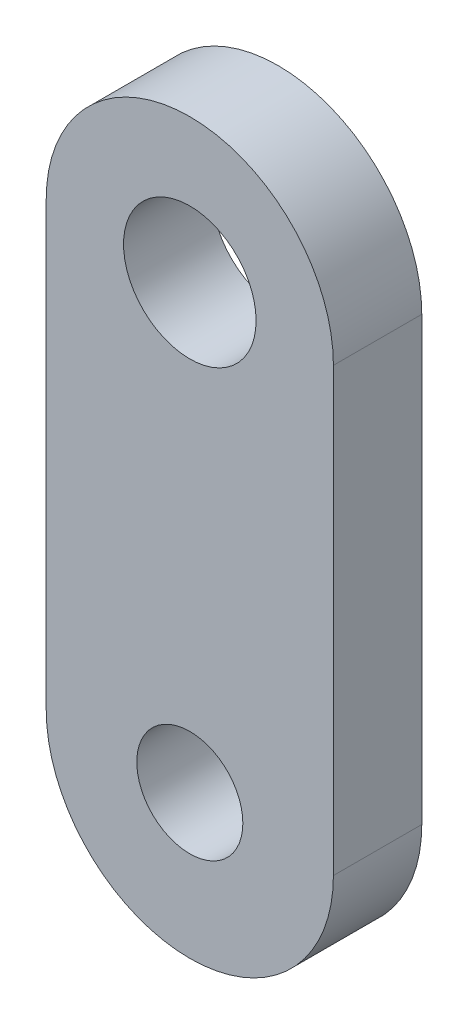
from build123d import *

# Parameters (mm, degrees)
SKETCH1_R           = 3
SKETCH1_R_2         = 2.4
BOSS_EXTRUDE1_DEPTH = 4


with BuildPart() as part:
    # Sketch1 → Boss-Extrude1 (new body)
    with BuildSketch(Plane.XY):
        with BuildLine():
            Line((6.5, 0), (6.5, -20))
            ThreePointArc((6.5, -20), (0, -26.5), (-6.5, -20))
            Line((-6.5, -20), (-6.5, 0))
            ThreePointArc((-6.5, 0), (0, 6.5), (6.5, 0))
        make_face()
        Circle(SKETCH1_R, mode=Mode.SUBTRACT)
        with Locations((0, -20)):
            Circle(SKETCH1_R_2, mode=Mode.SUBTRACT)
    extrude(amount=BOSS_EXTRUDE1_DEPTH)


solid = part.part
